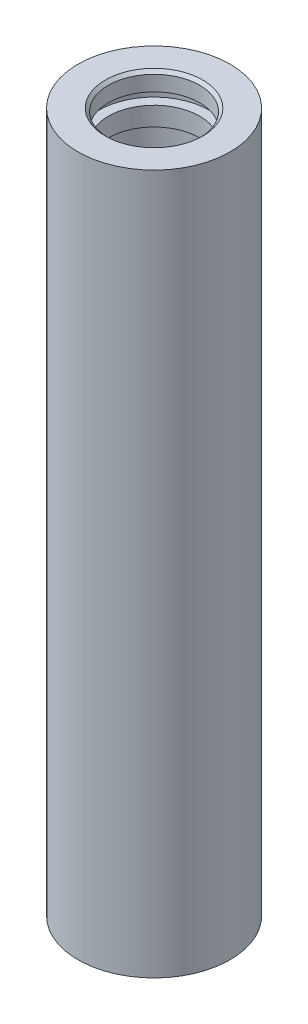
from build123d import *

# Parameters (mm, degrees)
CHAMFER_1_SIZE = 1


with BuildPart() as part:
    # 草图1 → 旋转1 (revolve)
    with BuildSketch(Plane.XY, mode=Mode.PRIVATE) as revolve_1_sk:
        Polygon((15, 6), (15, 0), (25, 0), (25, 230), (15, 230), (15, 224), (18.27, 224), (18.27, 220.2), (15, 220.2), (15, 214), (18, 214), (18, 16), (15, 16), (15, 9.8), (18.27, 9.8), (18.27, 6), align=None)
    revolve(revolve_1_sk.sketch.rotate(Axis((0, 0, 0), (0, 1, 0)), 90), axis=Axis((0, 0, 0), (0, 1, 0)))

    # 倒角1
    chamfer_1_edges = [part.edges().sort_by_distance(p)[0] for p in [
        (0, 230, 15),
        (0, 0, 15),
    ]]
    chamfer(chamfer_1_edges, length=CHAMFER_1_SIZE)


solid = part.part
